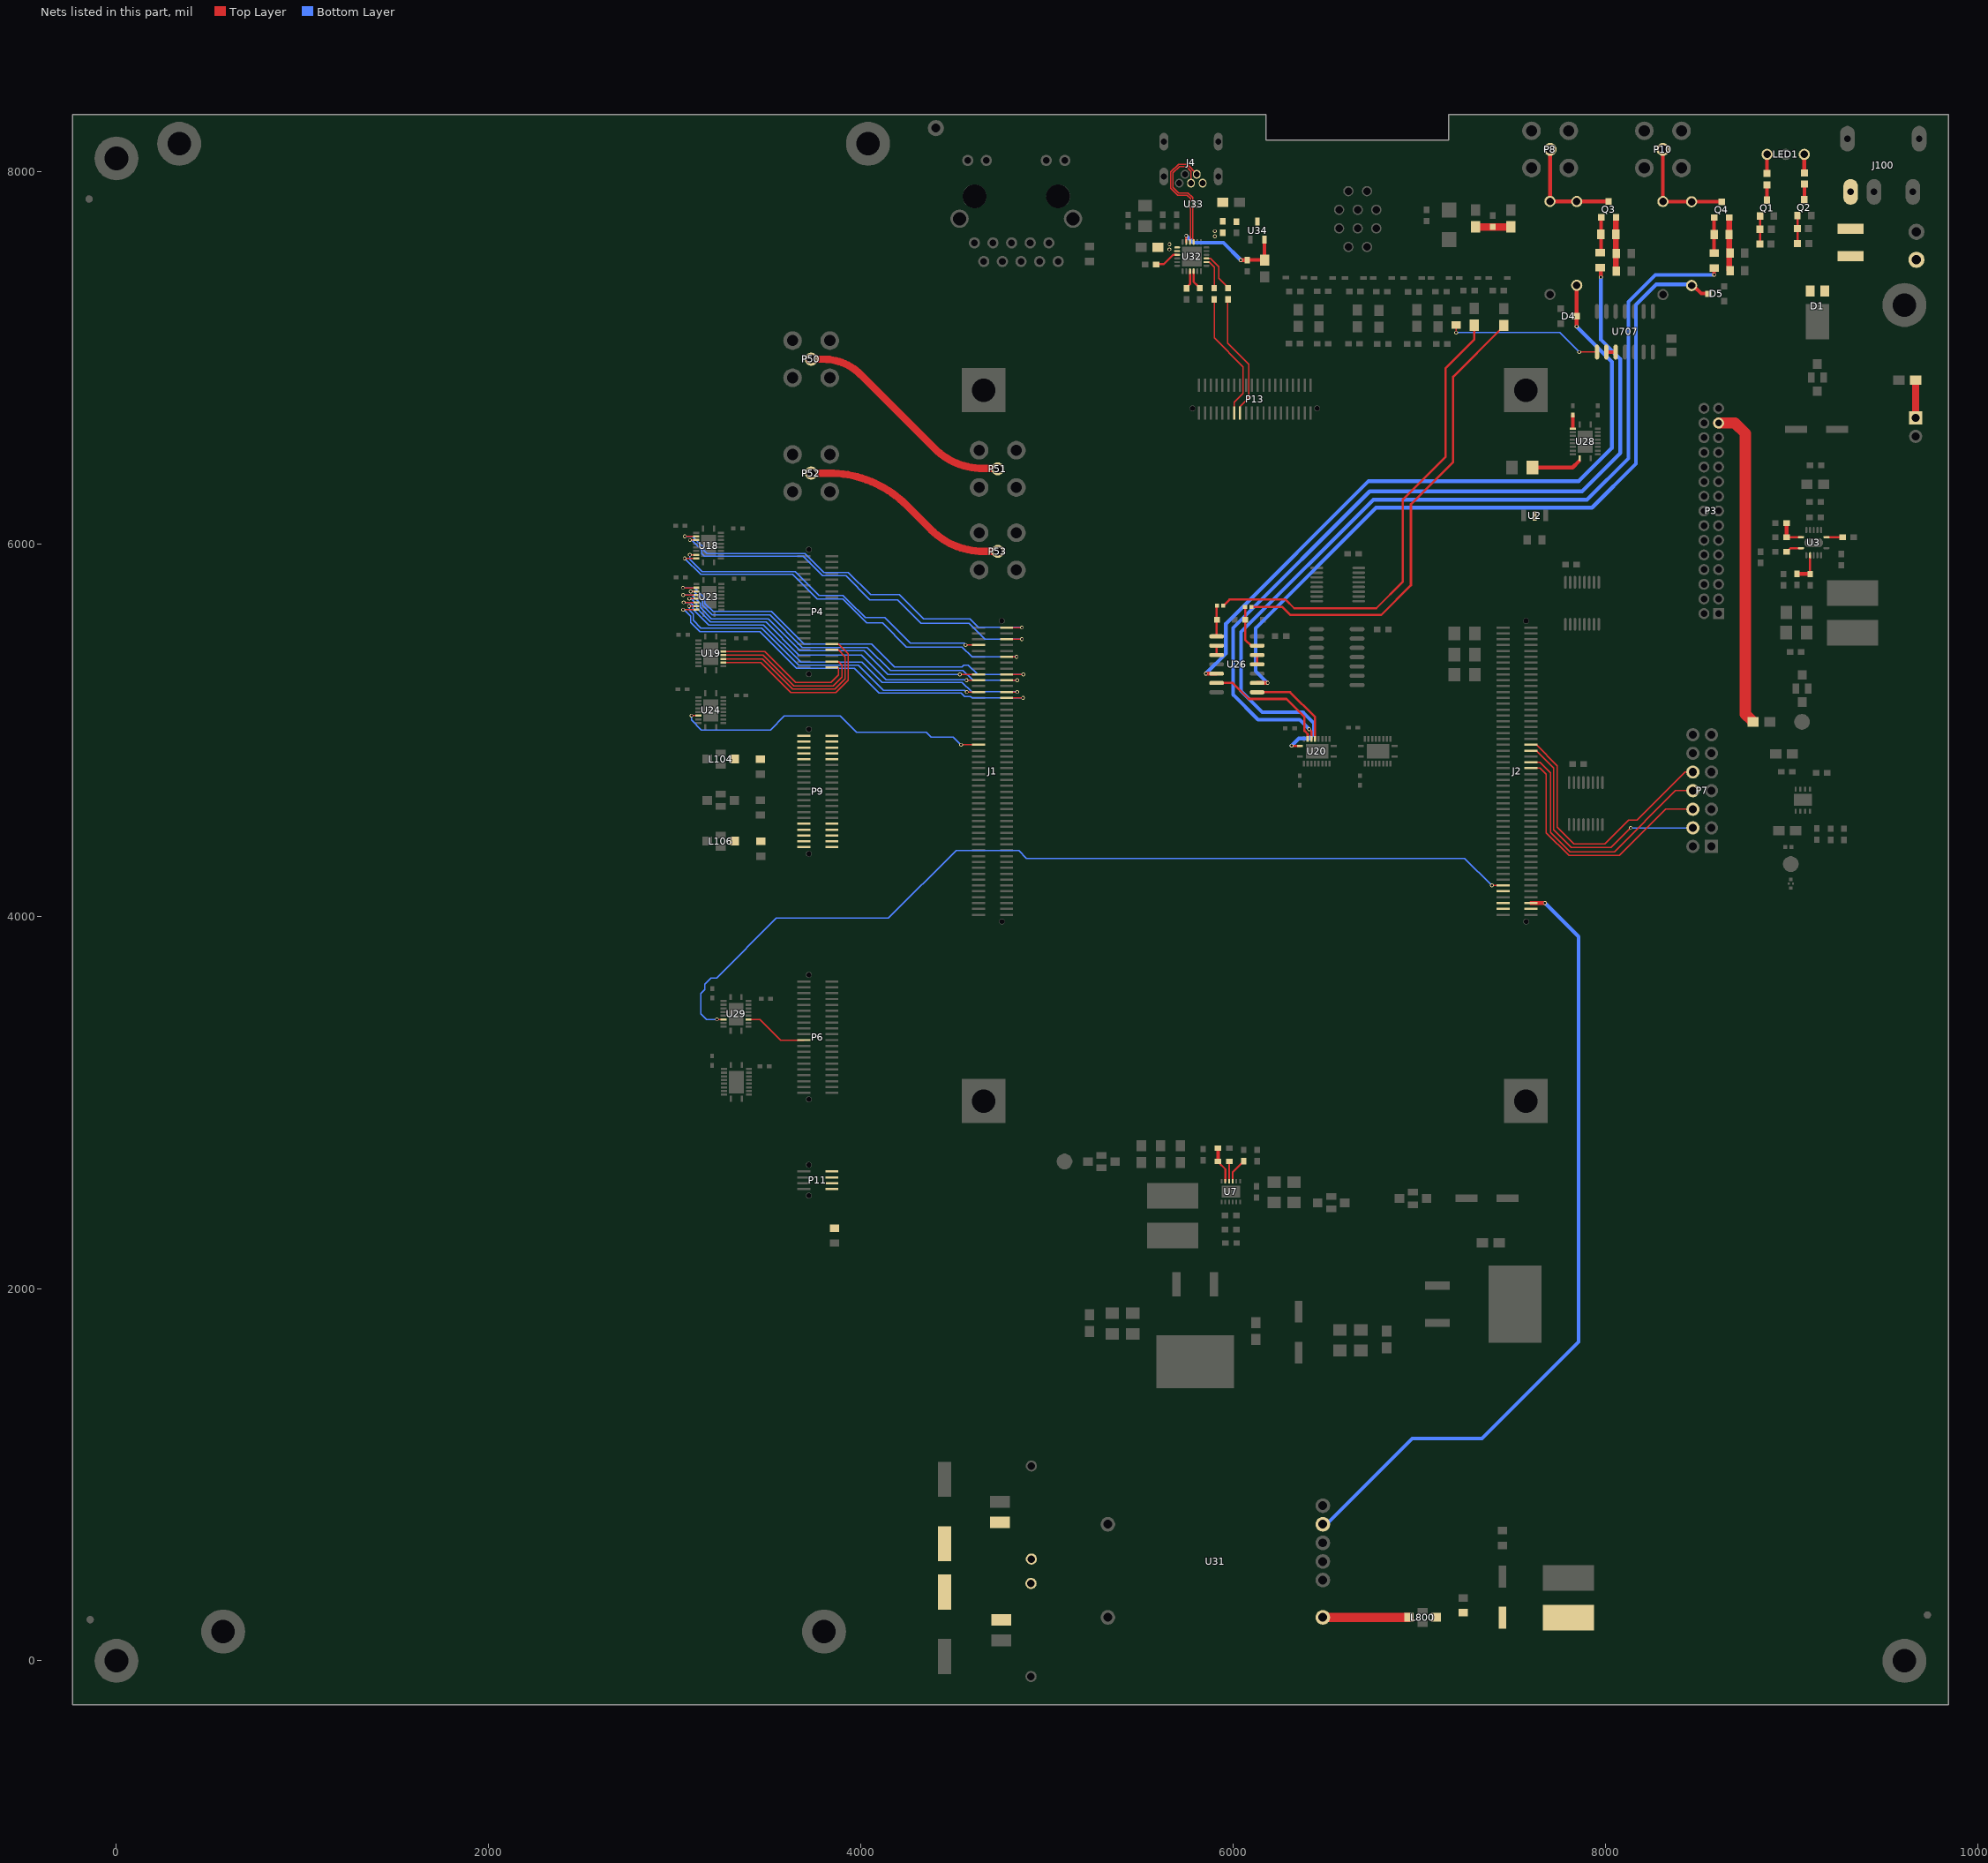
[diagram p0: the nets of this part, all layers, seen from the top]
# Altium PCB MISC82191.PcbDoc (part 8 of 9)
Units mil, origin at the board's own origin, x right, y up, seen from the top; angles counter-clockwise.
Board outline 10078.74 x 8543.31 mil, 4 copper layers (Top Layer, GND, POWER, Bottom Layer); 238 components, 299 nets, 1297 pads, 1665 vias.

## Via types
v1: diameter 20, hole 12, Top Layer to Bottom Layer, 1664 vias
v2: diameter 40, hole 20, Top Layer to Bottom Layer, 1 vias

## Nets (pads, with @x,y where several pads share a name; then routed paths per layer and width w, separated by ;. In a path a pad name is that pad's centre, name@x,y a point inside that pad or via, vN(x,y) a via of type N, cw(c..) or ccw(c..) an arc to the next point about the centre after c; other vN are vias at no path point) (continued)
NetC67_2: C67.2 F1.1 L19.1 | length 179
  Top Layer w40: L19.1@7302.78,7703.16 C67.2@7394.78,7703.16 F1.1@7481.78,7703.16
NetC91_1: C91.1 Q3.2 R35.1 R36.1 | length 284
  Top Layer w30: R35.1@8055.78,7466.16 R36.1@8055.78,7663.16 Q3.2@8055.78,7750.16
NetC92_2: C92.2 Q3.1 R36.2 | length 182
  Top Layer w20: C92.2@7976.78,7573.16 Q3.1@7976.78,7755.16
NetC95_1: C95.1 Q4.2 R39.1 R40.1 | length 282
  Top Layer w30: R39.1@8664.78,7471.16 Q4.2@8664.78,7753.16
NetC96_2: C96.2 Q4.1 R40.2 | length 181
  Top Layer w20: C96.2@8583.78,7562.16 R40.2@8583.78,7661.16 Q4.1@8583.78,7743.16
NetC97_1: C97.1 L106.1 P9.31 P9.32 P9.33 P9.34 P9.35 P9.36 P9.37 P9.38 P9.39 P9.40
NetC98_2: C98.2 C99.2 C101.1 C103.1 R43.1 R44.2
NetC100_1: C100.1 C102.1 L20.2 L800.1
NetC105_1: C105.1 FB1.2 U32.7 U32.8
  other v1: 5656.78,7582.16 5657.78,7610.16 5900.78,7652.16 5900.78,7680.16
NetC107_2: C107.2 U32.16 | length 88.8
  Top Layer w11: U32.16@5787.41,7464.68 5787.41,7417.16 5787.41,7407.53 C107.2@5809.78,7385.16
NetC704_2: C704.2 L104.1 P9.1 P9.2 P9.3 P9.4 P9.5 P9.6 P9.7 P9.8 P9.9 P9.10
NetCN1_1: CN1.1 R6.2 | length 186.7
  Top Layer w40: CN1.1@9666.52,6692.42 R6.2@9666.52,6879.09
NetD1_1: D1.1 D1.2 F2.2
NetD2_2: D2.2 R23.2 U26.1 | length 165
  Top Layer w6: R23.2@5912.74,5666.16 R23.2@5912.74,5668.16
  Top Layer w12: U26.1@5910.78,5503.16 R23.2@5910.78,5666.16
NetD3_2: D3.2 R34.1 U26.13 | length 256.3
  Top Layer w6: R34.1@6063.74,5655.16 R34.1@6063.74,5662.16
  Top Layer w12: R34.1@6063.78,5656.16 6063.78,5592.16 6063.78,5485.16 6095.78,5453.16 U26.13@6128.82,5453.16
NetF2_1: F2.1 J100.1 J300.1
NetF3_1: F3.1 P3.27 | length 1724.7
  Top Layer w60: P3.27@8607.78,6649.41 8695.78,6649.41 8751.78,6593.41 8751.78,5085.41 F3.1@8786.78,5050.41
NetL80(NC)_1: L80(NC).1 U707.8 | length 837.9
  Top Layer w6: v1(7197.4,7134.79) 7197.4,7175.09 ; v1(7858.78,7030.41) U707.8@7951.78,7030.41
  Bottom Layer w6: v1(7197.4,7134.79) 7754.4,7134.79 v1(7858.78,7030.41)
NetL800_3: L800.3 U31.5 | length 440.3
  Top Layer w50: U31.5@6503.78,233.41 L800.3@6944.11,233.41
NetLED1_1: LED1.1 R20.2 | length 92.1
  Top Layer w20: R20.2@8868.33,7989.36 LED1.1@8868.33,8081.47
NetLED1_3: LED1.3 R19.2 | length 76.1
  Top Layer w20: R19.2@9068.33,7993.36 LED1.3@9068.33,8069.47
NetP8_5: P8.5 Q3.3 R37.2 R38.2 | length 573
  Top Layer w20: R38.2@7701.78,7840.16 Q3.3@8005.78,7840.16 ; R38.2@7702.78,7850.16 P8.5@7702.78,8119.16
NetP10_5: P10.5 Q4.3 R41.2 R42.2 | length 573
  Top Layer w20: R42.2@8308.78,7857.16 P10.5@8308.78,8119.16 ; R42.2@8313.78,7838.16 R41.2@8462.78,7838.16 Q4.3@8624.78,7838.16
NetP11_2: P11.2 P11.4 P11.6 P11.8 RZ2.2
NetP50_5: P50.5 P51.5 | length 1221.5
  Top Layer w40: P50.5@3732.78,6992.41 3797.12,6992.41 cw(c3797.12,6705.94) 3999.69,6908.5 4394.85,6513.34 ccw(c4656.02,6774.51) 4656.02,6405.16 P51.5@4731.78,6405.16 ; P51.5@4731.78,6405.16 cw(c4731.78,6402.74) 4733.49,6404.45 P51.5@4734.78,6403.16 cw(c4734.78,6405.57) 4733.07,6403.86 P51.5@4731.78,6405.16
NetP52_5: P52.5 P53.5 | length 1129.6
  Top Layer w40: P52.5@3732.78,6380.6 3827.2,6380.6 cw(c3827.2,5788.79) 4245.67,6207.26 4376.42,6076.51 ccw(c4657.33,6357.42) 4657.33,5960.16 P53.5@4730.78,5960.16
NetQ1_1: Q1.1 R26.2 R28.2 | length 143.4
  Top Layer w12: R26.2@8830.4,7605.1 Q1.1@8830.4,7748.54
NetQ1_3: Q1.3 R20.1 | length 73.6
  Top Layer w20: Q1.3@8867.83,7847.36 R20.1@8867.83,7920.97
NetQ2_1: Q2.1 R25.2 R27.2 | length 144.4
  Top Layer w12: R25.2@9032.4,7612.1 Q2.1@9032.4,7756.54
NetQ2_3: Q2.3 R19.1 | length 74.6
  Top Layer w20: Q2.3@9068.83,7848.36 R19.1@9068.83,7922.97
NetR2_2: R2.2 R5.1 U3.10 | length 160
  Top Layer w11: R5.1@9099.18,5844.76 U3.10@9099.18,5938.72
  Top Layer w20: R2.2@9028.78,5839.16 R5.1@9094.78,5839.16
NetR4_1: R4.1 R7.1 U3.7 | length 141.3
  Top Layer w11: R4.1@8981.66,6036.28 U3.7@9050.96,6036.28
  Top Layer w20: R4.1@8972.78,6039.16 R7.1@8972.78,6111.16
NetR8_1: R8.1 U3.1 | length 79
  Top Layer w11: U3.1@9186.78,6036.16 R8.1@9265.78,6036.16
NetR9_1: R9.1 U3.8 | length 74.1
  Top Layer w11: R9.1@8981.78,5965.16 8993.72,5977.1 U3.8@9050.96,5977.1
NetR12_2: R12.2 U7.3 | length 124.5
  Top Layer w10: U7.3@5997.22,2575.83 5997.22,2624.6 R12.2@6050.78,2678.16
NetR13_1: R13.1 R14.1 U7.5 | length 182.3
  Top Layer w10: R13.1@5922.78,2676.16 5957.85,2641.09 U7.5@5957.85,2575.83
  Top Layer w20: R13.1@5918.59,2686.35 R14.1@5918.59,2753.83
NetR13_2: R13.2 U7.4 | length 101.1
  Top Layer w10: U7.4@5977.54,2575.83 R13.2@5977.54,2676.92
NetR45_1: R45.1 U32.21 | length 208.5
  Top Layer w6: U32.21@5856.32,7533.57 5877.37,7533.57 5921.78,7489.16 5921.78,7428.16 R45.1@5966.78,7383.16
NetR46_1: R46.1 U32.20 | length 156.9
  Top Layer w6: U32.20@5856.32,7513.88 5870.06,7513.88 5897.78,7486.16 R46.1@5897.78,7382.16
NetR47_1: R47.1 U32.9 | length 125.8
  Top Layer w11: R47.1@5593.78,7503.16 5627.78,7503.16 5677.87,7553.25 U32.9@5698.85,7553.25
NetR48_1: R48.1 U32.15 | length 90.7
  Top Layer w11: R48.1@5752.78,7380.16 5767.74,7395.11 U32.15@5767.74,7464.68
NetU26_2: U26.2 U26.3 | length 43
  Top Layer w12: U26.3@5910.78,5403.16 U26.2@5910.78,5446.16
NetU26_11: U26.11 U26.12 | length 50
  Top Layer w12: U26.11@6128.82,5353.16 U26.12@6128.82,5403.16
NetU707_9: U707.9 U707.10 | length 43.3
  Top Layer w20: U707.9@8004.78,7030.74 U707.10@8048.11,7030.74
OUTA: J2.B48
OUTB: J2.B49
OUTC: J2.A49
OUTD: J2.A48 U31.2 | length 4287.5
  Top Layer w20: J2.A48@7599.01,4070.69 v1(7675.24,4070.69)
  Bottom Layer w20: U31.2@6481.59,733.83 U31.2@6502.78,733.83 ; U31.2@6502.78,735.41 6961.78,1194.41 7336.78,1194.41 7855.78,1713.41 7855.78,3890.78 v1@7675.78,4070.78
S1: J1.A13 U23.9 | length 2354.2
  Top Layer w6: v1(3044.95,5646.33) U23.9@3116.38,5646.33 ; J1.A13@4782.37,5173.03 v1(4870.65,5173.03)
  Bottom Layer w6: v1(3044.95,5646.33) v1@3047.45,5643.83 ; v1@3049.78,5646.16 3084.78,5611.16 3084.78,5579.16 3135.78,5528.16 3457.03,5528.16 3653.03,5332.16 3784.78,5332.16 ; 3909.78,5332.16 3784.78,5332.16 ; 4851.65,5173.16 4821.78,5173.16 ; v1@4870.78,5172.16 4869.78,5173.16 4821.78,5173.16 ; 3784.78,5332.16 3964.03,5332.16 4097.03,5199.16 4538.78,5199.16 4556.78,5181.16 4588.78,5181.16 4596.78,5173.16 4821.78,5173.16
S2: J1.B12 U23.8 | length 1827.8
  Top Layer w6: v1(3076.64,5666.02) U23.8@3116.38,5666.02 ; v1(4568.15,5204.53) J1.B12@4632.75,5204.53
  Bottom Layer w6: v1@3076.64,5664.16 v1(3076.64,5666.02) ; v1@3078.78,5664.16 3078.78,5644.16 3099.78,5623.16 3099.78,5589.16 3140.78,5548.16 3467.03,5548.16 3667.03,5348.16 3914.78,5348.16 ; 3924.78,5348.16 3914.78,5348.16 ; v1@4567.78,5203.16 4556.78,5214.16 4120.03,5214.16 3986.03,5348.16 3914.78,5348.16
S3: J1.A12 U23.7 | length 2149.8
  Top Layer w6: v1(3047.24,5685.7) U23.7@3116.38,5685.7 ; J1.A12@4782.37,5204.53 v1(4839.41,5204.53)
  Bottom Layer w6: v1(3047.24,5685.7) 3083.82,5685.7 3097.78,5671.74 3097.78,5649.16 3181.78,5565.16 3476.78,5565.16 3676.78,5365.16 3923.78,5365.16 ; 3943.78,5365.16 3923.78,5365.16 ; v1@4837.78,5203.16 4835.78,5205.16 4594.78,5205.16 4543.78,5256.16 4115.03,5256.16 4006.03,5365.16 3923.78,5365.16
S4: J1.B10 U23.6 | length 1809.3
  Top Layer w6: v1(3078.01,5705.39) U23.6@3116.38,5705.39 ; v1(4567.42,5267.52) J1.B10@4632.75,5267.52
  Bottom Layer w6: v1(3078.01,5705.39) 3087.55,5705.39 3118.78,5674.16 3118.78,5653.16 3191.78,5580.16 3490.78,5580.16 3666.78,5404.16 3927.78,5404.16 ; 3939.78,5404.16 3927.78,5404.16 ; 4548.42,5271.16 4535.78,5271.16 ; v1@4564.78,5266.16 4559.78,5271.16 4535.78,5271.16 ; 3927.78,5404.16 4002.03,5404.16 4135.03,5271.16 4535.78,5271.16
S5: J1.B9 U23.5 | length 1862.1
  Top Layer w6: v1(3044.69,5725.07) U23.5@3116.38,5725.07 ; v1(4530.92,5299.01) J1.B9@4632.75,5299.01
  Bottom Layer w6: v1(3044.69,5725.07) 3091.87,5725.07 3136.78,5680.16 3136.78,5658.16 3196.78,5598.16 3501.78,5598.16 3672.78,5427.16 3936.78,5427.16 ; 3949.78,5427.16 3936.78,5427.16 ; v1(4530.92,5299.01) 4145.18,5299.01 4017.03,5427.16 3936.78,5427.16
S9: J1.A6 U18.9 | length 2180.1
  Top Layer w6: v1(3052.95,5922.33) U18.9@3114.28,5922.33 ; J1.A6@4782.37,5393.5 v1(4836.12,5393.5)
  Bottom Layer w6: v1(3052.95,5922.33) 3139.13,5836.16 3632.78,5836.16 3764.78,5704.16 3902.03,5704.16 4030.78,5575.41 4115.78,5575.41 4245.03,5446.16 4543.78,5446.16 4596.78,5393.16 4744.78,5393.16 ; 4814.78,5393.16 4744.78,5393.16 ; v1@4828.78,5393.16 4744.78,5393.16
S10: J1.B4 U18.8 | length 1812.2
  Top Layer w6: v1(3080.64,5942.02) U18.8@3114.28,5942.02 ; v1(4562.44,5456.49) J1.B4@4632.75,5456.49
  Bottom Layer w6: v1(3080.64,5942.02) 3080.64,5917.3 3145.78,5852.16 3646.78,5852.16 3774.78,5724.16 3902.78,5724.16 3932.15,5694.78 ; 3940.78,5686.16 3932.15,5694.78 ; v1@4561.78,5458.16 4553.78,5466.16 4265.03,5466.16 4127.78,5603.41 4023.53,5603.41 3932.15,5694.78
S11: J1.A9 U23.3 | length 2206
  Top Layer w6: v1(3043.78,5764.16) 3044.78,5764.16 3045.06,5764.44 U23.3@3116.38,5764.44 ; J1.A9@4782.37,5299.01 v1(4872.64,5299.01)
  Bottom Layer w6: v1(3043.78,5764.16) 3106.78,5764.16 3161.78,5709.16 3161.78,5681.16 3205.78,5637.16 3518.78,5637.16 3693.78,5462.16 4058.03,5462.16 4181.03,5339.16 4512.78,5339.16 4542.78,5339.16 4553.13,5349.51 4576.43,5349.51 4627.78,5298.16 v1@4868.78,5298.16
S12: J1.A10 U23.4 | length 2061.8
  Top Layer w6: v1(3084.78,5744.16) 3085.38,5744.76 U23.4@3116.38,5744.76 ; J1.A10@4782.37,5267.52 v1(4839.14,5267.52)
  Bottom Layer w6: v1(3084.78,5744.16) 3100.78,5744.16 3148.78,5696.16 3148.78,5671.16 3201.78,5618.16 3511.78,5618.16 3685.78,5444.16 3953.78,5444.16 ; 3962.78,5444.16 3953.78,5444.16 ; v1@4836.78,5267.16 4601.78,5267.16 4548.78,5320.16 4158.03,5320.16 4034.03,5444.16 3953.78,5444.16
S13: J1.A3 U18.4 | length 2139.9
  Top Layer w6: v1(3081.18,6020.76) U18.4@3114.28,6020.76 ; J1.A3@4782.37,5487.99 v1(4864.61,5487.99)
  Bottom Layer w6: v1(3081.18,6020.76) 3090.18,6020.76 3143.78,5967.16 3143.78,5949.16 3159.78,5933.16 3690.78,5933.16 3794.78,5829.16 3919.78,5829.16 4048.53,5700.41 4196.78,5700.41 4323.03,5574.16 4579.78,5574.16 4665.78,5488.16 4836.78,5488.16 ; 4845.61,5488.16 4836.78,5488.16 ; v1@4865.78,5488.16 4836.78,5488.16
S14: J1.A1 U18.3 | length 2176.6
  Top Layer w6: v1(3053.5,6040.44) U18.3@3114.28,6040.44 ; J1.A1@4782.37,5550.98 v1(4864.6,5550.98)
  Bottom Layer w6: v1(3053.5,6040.44) 3094.5,6040.44 3155.78,5979.16 3155.78,5964.16 3171.78,5948.16 3699.78,5948.16 3800.78,5847.16 3931.78,5847.16 4051.53,5727.41 4205.78,5727.41 4336.03,5597.16 4585.78,5597.16 4631.78,5551.16 4834.78,5551.16 ; 4845.6,5551.16 4834.78,5551.16 ; v1@4864.78,5551.16 4834.78,5551.16
S15: J1.B21 U24.7 | length 1720.6
  Top Layer w6: v1(3089.24,5077.7) U24.7@3126.38,5077.7 ; v1(4537.85,4921.09) J1.B21@4632.75,4921.09
  Bottom Layer w6: v1(3089.24,5077.7) 3089.24,5053.7 3142.78,5000.16 3513.78,5000.16 3588.78,5075.16 3889.03,5075.16 3975.41,4988.78 4351.15,4988.78 4377.78,4962.16 4495.78,4962.16 v1@4536.78,4921.16
T+: J2.B45 U29.7 | length 4944.6
  Top Layer w6: v1(3226.24,3445.7) U29.7@3262.38,3445.7 ; v1(7389.78,4165.16) J2.B45@7428.78,4165.16
  Bottom Layer w6: v1(3226.24,3445.7) 3171.24,3445.7 3140.78,3476.16 3140.78,3584.16 3161.78,3605.16 3161.78,3635.16 3195.28,3668.66 3225.28,3668.66 3545.91,3989.28 4147.65,3989.28 4511.53,4353.16 4848.03,4353.16 4889.78,4311.41 7243.53,4311.41 v1(7389.78,4165.16) v1@7389.4,4165.16
T-: J2.B46
TCK: J2.A25 P7.6 | length 1351.6
  Top Layer w6: J2.A25@7599.01,4795.1 7648.84,4795.1 7681.78,4762.16 7681.78,4448.41 7803.78,4326.41 8075.78,4326.41 8324.15,4574.78 P7.6@8469.78,4574.78
TDI: J2.A21 P7.10 | length 1446.6
  Top Layer w6: J2.A21@7599.01,4921.09 7628.85,4921.09 7740.78,4809.16 7740.78,4477.41 7830.78,4387.41 7995.78,4387.41 8125.78,4517.41 8169.78,4517.41 8427.15,4774.78 P7.10@8469.78,4774.78
TDO: J2.A24 P7.8 | length 1393
  Top Layer w6: J2.A24@7599.01,4826.6 7649.34,4826.6 7705.78,4770.16 7705.78,4450.41 7809.78,4346.41 8047.78,4346.41 8376.15,4674.78 P7.8@8469.78,4674.78
TMS: J2.A22 P7.4 | length 1324
  Top Layer w6: J2.A22@7599.01,4889.59 7628.35,4889.59 7722.78,4795.16 7722.78,4463.41 7816.78,4369.41 8029.78,4369.41 v1@8135.15,4474.78
  Bottom Layer w6: v1(8135.41,4474.78) P7.4@8469.78,4474.78
TRIGGER1_IN: D4.3 R37.1 U26.5 | length 3778.5
  Top Layer w20: v1(5852.78,5303.16) U26.5@5910.78,5303.16 ; v1(7844.78,7168.16) D4.3@7844.78,7223.16 R37.1@7844.78,7379.16
  Bottom Layer w20: v1(5852.78,5303.16) 5960.78,5411.16 5960.78,5571.16 6727.03,6337.41 7857.03,6337.41 8034.78,6515.16 8034.78,6978.16 v1(7844.78,7168.16)
TRIGGER1_IN+: U20.18 U26.6 | length 681.9
  Top Layer w12: U26.6@5909.78,5253.16 U26.6@5910.78,5253.16 5997.78,5253.16 6083.78,5167.16 6285.78,5167.16 6382.78,5070.16 6382.78,4996.16 6400.14,4978.8 U20.18@6400.14,4953.18 U20.18@6400.14,4962.16
TRIGGER1_OUT: C92.1 U20.17 | length 4407.2
  Top Layer w12: v1(6407.78,5005.16) 6419.83,4993.11 U20.17@6419.83,4953.18
  Top Layer w20: v1(7975.78,7433.16) C92.1@7975.78,7484.16
  Bottom Layer w20: v1@6406.78,5006.16 6356.78,5056.16 6133.78,5056.16 5999.78,5190.16 5999.78,5549.16 6733.03,6282.41 7874.03,6282.41 8079.78,6488.16 8079.78,6993.16 7975.78,7097.16 v1(7975.78,7433.16)
TRIGGER2_IN: D5.3 R41.1 U26.9 | length 4070.4
  Top Layer w20: U26.9@6128.82,5253.16 v1(6184.78,5253.16) ; R41.1@8479.78,7380.16 8514.85,7345.09 8544.85,7345.09 D5.3@8545.78,7344.16
  Bottom Layer w20: v1(6184.78,5253.16) 6120.78,5317.16 6120.78,5547.16 6768.03,6194.41 7863.78,6194.41 7928.03,6194.41 8163.78,6430.16 8163.78,7285.16 8272.78,7394.16 8453.78,7394.16 R41.1@8463.78,7384.16
TRIGGER2_IN+: U20.16 U26.8 | length 482.3
  Top Layer w12: U26.8@6128.82,5203.16 6305.78,5203.16 6439.51,5069.43 U20.16@6439.51,4953.18
TRIGGER2_OUT: C96.1 U20.20 | length 4894.1
  Top Layer w12: v1@6314.16,4915.78 U20.20@6358.8,4915.78
  Top Layer w20: v1(8583.78,7445.16) C96.1@8583.78,7482.16
  Bottom Layer w20: v1(6313.78,4916.16) 6352.78,4955.16 6409.78,4955.16 6433.78,4979.16 6433.78,5037.16 6374.78,5096.16 6155.78,5096.16 6042.78,5209.16 6042.78,5527.16 6753.03,6237.41 7901.03,6237.41 8122.78,6459.16 8122.78,7300.16 8267.78,7445.16 v1(8583.78,7445.16)
TT: P6.21 U29.14 | length 343.9
  Top Layer w6: U29.14@3396.24,3445.7 3457.24,3445.7 3568.12,3334.82 P6.21@3694.21,3334.82
U15_IN1: P4.40 U19.16 | length 777.1
  Top Layer w6: U19.16@3260.24,5422.07 3482.87,5422.07 3648.78,5256.16 3839.78,5256.16 3879.78,5296.16 3879.78,5330.16 3874.1,5335.83 P4.40@3843.82,5335.83
U15_IN2: P4.38 U19.15 | length 850.8
  Top Layer w6: U19.15@3260.24,5402.39 3474.55,5402.39 3639.78,5237.16 3849.78,5237.16 3897.78,5285.16 3897.78,5348.16 3878.61,5367.33 P4.38@3843.82,5367.33
U15_IN3: P4.34 U19.14 | length 948.2
  Top Layer w6: U19.14@3260.24,5382.7 3471.24,5382.7 3632.78,5221.16 3859.78,5221.16 3914.78,5276.16 3914.78,5394.16 3878.61,5430.32 P4.34@3843.82,5430.32
U15_IN4: P4.32 U19.13 | length 1018.3
  Top Layer w6: U19.13@3260.24,5363.02 3460.92,5363.02 3622.78,5201.16 3865.78,5201.16 3931.78,5267.16 3931.78,5410.16 3880.12,5461.82 P4.32@3843.82,5461.82
UART_RXD: P13.13 R46.2 | length 688.1
  Top Layer w6: R46.2@5897.78,7307.16 5897.78,7106.16 6052.78,6951.16 6052.78,6808.16 6005.65,6761.02 P13.13@6005.65,6702.82
UART_TXD: P13.15 R45.2 | length 672.5
  Top Layer w6: R45.2@5970.78,7309.16 5970.78,7078.16 6083.78,6965.16 6083.78,6785.16 6037.14,6738.52 P13.15@6037.14,6702.82
USB_5VIN: C104.2 C109.2 FB1.1 J4.1 U34.3
USB_UART_D+: J4.3 U32.3 U33.2 U33.5 | length 626.9
  Top Layer w6: J4.3@5769.78,7940.16 5773.92,7944.3 5773.92,7947.3 5773.92,8002.05 5748.81,8027.16 5710.75,8027.16 5677.18,7993.59 5677.18,7915.73 5707.75,7885.16 5757.78,7885.16 5782.62,7860.32 5782.62,7846.32 5786.46,7842.47 U33.5@5786.46,7836.78 U33.2@5786.46,7815.84 ; U33.2@5786.78,7809.16 5783.57,7805.95 5783.57,7638.36 5787.41,7634.53 U32.3@5787.41,7622.16
USB_UART_D-: J4.2 U32.4 U33.1 U33.6 | length 629.8
  Top Layer w6: U33.1@5766.78,7815.16 U33.6@5766.78,7836.78 5766.78,7842.16 5770.62,7846 5770.62,7855.34 5752.81,7873.16 5702.78,7873.16 5665.18,7910.76 5665.18,7998.56 5705.78,8039.16 5753.78,8039.16 5802.78,7990.16 J4.2@5802.78,7983.16 ; U32.4@5767.74,7622.16 5767.74,7634.11 5771.57,7637.95 5771.57,7805.36 U33.1@5767.78,7809.16
VCC1V8: C3.1 C88.2 U2.2 U28.2 U28.10 | length 330.1
  Top Layer w20: C3.1@7607.78,6410.16 7823.78,6410.16 U28.10@7857.78,6444.16 ; 7824.78,6626.16 C88.2@7824.78,6692.16
VCC1V8U: C108.2 C110.2 U32.5 U34.2 | length 595.8
  Top Layer w12: U32.5@5748.04,7622.16 v1(5748.04,7654.9)
  Top Layer w20: v1(6040.78,7524.16) C108.2@6069.78,7524.16 ; C108.2@6085.78,7525.16 6161.39,7525.16 6167.58,7531.35 U34.2@6167.58,7634.16
  Bottom Layer w20: v1(5748.04,7654.9) 5784.78,7618.16 5946.78,7618.16 v1(6040.78,7524.16)
"ZERO A": L12.1 R23.1 | length 2591.7
  Top Layer w6: R23.1@5943.78,5670.16 R23.1@5944.3,5670.68 ; L12.1@7295.78,7165.16 L12.1@7295.78,7172.16
  Top Layer w12: R23.1@5946.82,5668.16 5979.82,5701.16 6280.78,5701.16 6327.78,5654.16 6768.78,5654.16 6911.78,5797.16 6911.78,6239.16 7141.78,6469.16 7141.78,6944.16 7294.78,7097.16 L12.1@7294.78,7165.16
"ZERO B": L11.1 R34.2 | length 2534.5
  Top Layer w6: L11.1@7440.78,7157.16 L11.1@7449.78,7166.16
  Top Layer w12: R34.2@6097.82,5662.16 6262.78,5662.16 6306.78,5618.16 6794.78,5618.16 6954.78,5778.16 6954.78,6213.16 7181.78,6440.16 7181.78,6898.16 L11.1@7440.78,7157.16
pads on no net: J1.0 J1.A19 J1.A43 J1.A49 J1.B24 J2.0 J4.0 J4.4 J100.4 J100.5 P4.0 P6.0 P6.1 P6.2 P6.3 P6.4 P6.7 P6.8 P6.9 P6.10 P6.13 P6.14 P6.15 P6.16 P6.26 P6.32 P7.1 P7.12 P7.14 P9.0 P11.0 P13.0 R12.1 RJ1. U3.14 U17.13 U17.14 U17.15 U18.1 U18.20 U19.1 U19.20 U20.15 U21.13 U21.14 U21.15 U22.13 U22.14 U22.15 U23.1 U23.20 U24.9 U24.12 U24.18 U24.20 U31.1 U31.3 U31.8 U32.1 U32.10 U32.11 U32.12 U32.13 U32.14 U32.17 U32.18 U32.19 U32.22 U32.23 U32.24 U707.1 U707.2 U707.3 U707.4 U707.5 U707.6 U707.12 U707.13

## Polygon pours and split planes (outlines as drawn)
13V on Top Layer "Bottom Layer-No Net" (solid, remove dead copper, pour order 1012): 19 vertices, not listed, extent 7646.78,374.41 7980.78,680.41
13V on Top Layer "Bottom Layer-No Net" (solid, remove dead copper, pour order 1011): 2939.78,4450.41 2939.78,4354.41 2949.78,4344.41 2975.78,4318.41 3029.78,4318.41 3179.78,4318.41 3196.78,4335.41 3200.78,4339.41 3200.78,4384.41 3200.78,4468.41 3194.78,4474.41 3188.78,4480.41 3156.78,4480.41 2969.78,4480.41 2939.78,4450.41
A6V on Top Layer "Bottom Layer-No Net" (solid, remove dead copper, pour order 1010): 65 vertices, not listed, extent 2658.78,1830.41 5724.78,4683.41
-5.4V on Top Layer "Bottom Layer-No Net" (solid, remove dead copper, pour order 1009): 18 vertices, not listed, extent 3029.78,4773.41 3200.78,4914.41
-5.4V on Top Layer "Bottom Layer-No Net" (solid, remove dead copper, pour order 1008): 18 vertices, not listed, extent 4908.78,2597.41 5246.78,2776.41
NetF2_1 on Top Layer "Bottom Layer-No Net" (solid, remove dead copper, pour order 1007): 42 vertices, not listed, extent 9190.78,7466.41 9733.78,7979.41
NetD1_1 on Top Layer "Bottom Layer-No Net" (solid, remove dead copper, pour order 1006): 18 vertices, not listed, extent 9064.78,7326.41 9420.78,7577.41
"9V 1.5A" on Top Layer "Bottom Layer-No Net" (solid, remove dead copper, pour order 1005): 42 vertices, not listed, extent 5860.78,1742.41 7166.78,2105.41
13V on Top Layer "Bottom Layer-No Net" (solid, remove dead copper, pour order 1004): 18 vertices, not listed, extent 6573.78,2369.41 6918.78,2555.41
NetC97_1 on Top Layer "Bottom Layer-No Net" (solid, remove dead copper, pour order 1003): 30 vertices, not listed, extent 3294.78,4363.41 3893.78,4504.41
A6V4 on Top Layer "Bottom Layer-No Net" (solid, remove dead copper, pour order 1002): 30 vertices, not listed, extent 3295.78,4586.41 3893.78,4724.41
NetC704_2 on Top Layer "Bottom Layer-No Net" (solid, remove dead copper, pour order 1001): 26 vertices, not listed, extent 3293.78,4817.41 3888.78,4976.41
D5V on Top Layer "Bottom Layer-No Net" (solid, remove dead copper, pour order 1000): 38 vertices, not listed, extent 8852.78,4667.41 9148.78,5177.41
13V on Top Layer "Bottom Layer-No Net" (solid, remove dead copper, pour order 1050): 19 vertices, not listed, extent 7264.78,5262.16 7739.78,5557.16
3V3 on Top Layer "Bottom Layer-No Net" (solid, remove dead copper, pour order 1106): 18 vertices, not listed, extent 8949.78,4081.16 9033.78,4161.16
3V3 on Top Layer "Bottom Layer-No Net" (solid, remove dead copper, pour order 1105): 22 vertices, not listed, extent 7637.78,5980.16 7753.78,6183.16
3V3 on Top Layer "Bottom Layer-No Net" (solid, remove dead copper, pour order 1104): 17 vertices, not listed, extent 5384.78,7748.16 5458.78,7831.16
13V on Top Layer "Bottom Layer-No Net" (solid, remove dead copper, pour order 1103): 34 vertices, not listed, extent 8964.78,6841.16 9604.78,7284.16
NetC12_2 on Top Layer "Bottom Layer-No Net" (solid, remove dead copper, pour order 1102): 40 vertices, not listed, extent 8949.78,4188.16 9226.78,4578.16
NetC8_1 on Top Layer "Bottom Layer-No Net" (solid, remove dead copper, pour order 1100): 37 vertices, not listed, extent 8933.78,6059.16 9214.78,6847.16
NetC17_1 on Top Layer "Bottom Layer-No Net" (solid, remove dead copper, pour order 1099): 30 vertices, not listed, extent 9021.78,5270.16 9480.78,5673.16
NetC11_2 on Top Layer "Bottom Layer-No Net" (solid, remove dead copper, pour order 1098): 34 vertices, not listed, extent 9112.78,5666.16 9479.78,5956.16
NetC98_2 on Top Layer "Bottom Layer-No Net" (solid, remove dead copper, pour order 1097): 27 vertices, not listed, extent 4378.78,184.16 4968.78,771.16
NetC23_1 on Top Layer "Bottom Layer-No Net" (solid, remove dead copper, pour order 1093): 30 vertices, not listed, extent 7014.4,1981.78 7367.4,2738.78
NetC41_1 on Top Layer "Bottom Layer-No Net" (solid, remove dead copper, pour order 1092): 26 vertices, not listed, extent 6031.78,2337.16 6479.78,2506.16
NetC44_1 on Top Layer "Bottom Layer-No Net" (solid, remove dead copper, pour order 1091): 29 vertices, not listed, extent 5472.78,2173.16 5976.78,2478.16
NetC47_2 on Top Layer "Bottom Layer-No Net" (solid, remove dead copper, pour order 1090): 25 vertices, not listed, extent 5339.78,2429.16 5943.78,2709.16
KGND on Top Layer "Bottom Layer-No Net" (solid, remove dead copper, pour order 1083): 35 vertices, not listed, extent 6734.78,7540.16 7200.78,7849.16
NetC105_1 on Top Layer "Bottom Layer-No Net" (solid, remove dead copper, pour order 1080): 5881.78,7683.16 5881.78,7647.16 5887.78,7641.16 5892.78,7636.16 5914.78,7636.16 5959.78,7636.16 5966.78,7643.16 5967.78,7644.16 5967.78,7683.16 5962.78,7688.16 5959.78,7691.16 5942.78,7691.16 5889.78,7691.16 5881.78,7683.16
NetC105_1 on Top Layer "Bottom Layer-No Net" (solid, remove dead copper, pour order 1077): 23 vertices, not listed, extent 5565.78,7567.16 5714.78,7636.16
C3.3V on Top Layer "Bottom Layer-No Net" (solid, remove dead copper, pour order 1075): 52 vertices, not listed, extent 5367.78,7459.16 5733.78,7739.16
USB_5VIN on Top Layer "Bottom Layer-No Net" (solid, remove dead copper, pour order 1073): 39 vertices, not listed, extent 5811.78,7712.16 6148.78,7962.16
NetC51_1 on Top Layer "Bottom Layer-No Net" (solid, remove dead copper, pour order 1049): 22 vertices, not listed, extent 5028.78,7465.16 5267.78,7553.16
VCC1V8 on Top Layer "Bottom Layer-No Net" (solid, remove dead copper, pour order 1047): 34 vertices, not listed, extent 7575.78,6117.16 7836.78,6704.16
D5V on Top Layer "Bottom Layer-No Net" (solid, remove dead copper, pour order 1046): 19 vertices, not listed, extent 7458.78,7761.16 7590.78,7829.16
HT on Top Layer "Bottom Layer-No Net" (solid, remove dead copper, pour order 1045): 49 vertices, not listed, extent 3551.78,673.78 5393.78,2636.78
KGND on Top Layer "Bottom Layer-No Net" (solid, remove dead copper, pour order 1056): 46 vertices, not listed, extent 4326.78,7577.78 5262.78,8281.78
NetC100_1 on Top Layer "Bottom Layer-No Net" (solid, remove dead copper, pour order 1000): 21 vertices, not listed, extent 7063.78,83.41 7954.78,304.41
NetP11_2 on Top Layer "Bottom Layer-No Net" (solid, remove dead copper, pour order 1001): 18 vertices, not listed, extent 3805.78,2304.41 3913.78,2638.41
HGND on Top Layer "Bottom Layer-No Net" (solid, remove dead copper, pour order 1002): 18 vertices, not listed, extent 3802.78,2137.41 3912.78,2265.41
HGND on Top Layer "Bottom Layer-No Net" (solid, remove dead copper, pour order 1003): 46 vertices, not listed, extent 6431.78,176.41 7505.78,640.41
HGND on Top Layer "Bottom Layer-No Net" (solid, remove dead copper, pour order 1004): 22 vertices, not listed, extent 4399.78,-136.59 5381.78,285.41
DGND on Top Layer "Bottom Layer-No Net" (solid, remove dead copper, pour order 1005): 53 vertices, not listed, extent -1001.22,516.41 10240.78,8712.41
KGND on Bottom Layer "Bottom Layer-No Net" (solid, remove dead copper, pour order 1108): 55 vertices, not listed, extent 5078.78,7287.16 7396.78,7837.16